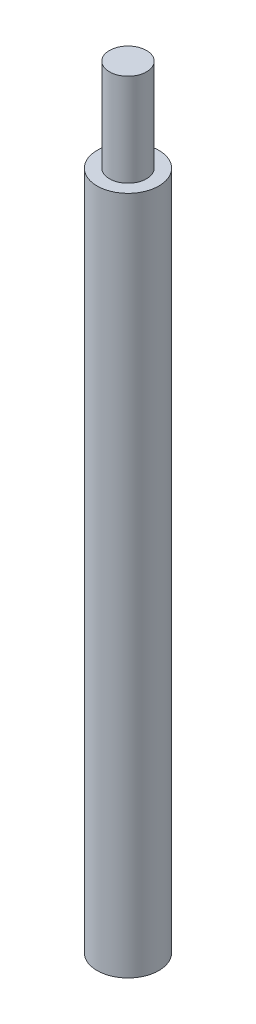
from build123d import *

# Parameters (mm, degrees)
SKETCH1_R           = 10
BOSS_EXTRUDE1_DEPTH = 250
SKETCH2_OUTSIDE_W   = 72.318
SKETCH2_OUTSIDE_H   = 72.318
SKETCH2_OUTSIDE_R   = 6
CUT_EXTRUDE1_DEPTH  = 30


with BuildPart() as part:
    # Sketch1 → Boss-Extrude1 (new body)
    with BuildSketch(Plane(origin=(0, 0, 0), x_dir=(1, 0, 0), z_dir=(0, 1, 0))):
        with Locations(Location((0, 0, 0), (0, 0, 270))):
            Circle(SKETCH1_R)
    extrude(amount=BOSS_EXTRUDE1_DEPTH)

    # Sketch2 outside → Cut-Extrude1 (cut)
    with BuildSketch(Plane(origin=(0, 250, 0), x_dir=(1, 0, 0), z_dir=(0, 1, 0))):
        Rectangle(SKETCH2_OUTSIDE_W, SKETCH2_OUTSIDE_H)
        with Locations(Location((0, 0, 0), (0, 0, 270))):
            Circle(SKETCH2_OUTSIDE_R, mode=Mode.SUBTRACT)
    extrude(amount=-CUT_EXTRUDE1_DEPTH, mode=Mode.SUBTRACT)


solid = part.part
